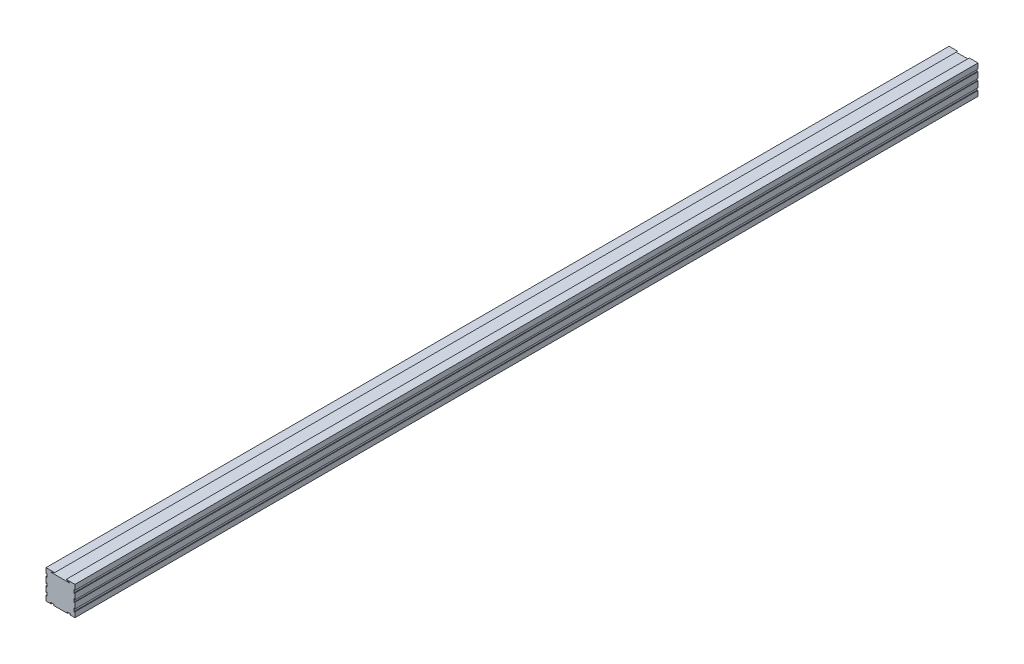
SolidWorks part; units mm, degrees
ref_plane "前视基准面" through (0, 0, 0) normal (0, 0, 1) x (1, 0, 0)
ref_plane "上视基准面" through (0, 0, 0) normal (0, 1, 0) x (1, 0, 0)
ref_plane "右视基准面" through (0, 0, 0) normal (1, 0, 0) x (0, 0, -1)
sketch "草图1" plane through (0, 0, 0) normal (0, 0, 1) x (1, 0, 0)
  line L1 (-37.5, 37.5) -> (37.5, 37.5)
  line L2 (-37.5, 37.5) -> (-37.5, -37.5)
  line L3 (-37.5, -37.5) -> (37.5, -37.5)
  line L4 (37.5, 37.5) -> (37.5, -37.5)
  line L5 (-37.5, 37.5) -> (37.5, -37.5) construction
  line L6 (-37.5, -37.5) -> (37.5, 37.5) construction
  point P0 (0, 0)
  dimension "D1" = 75
  dimension "D2" = 75
extrude "凸台-拉伸1" add sketch "草图1" along normal mid plane 2340 contours L1 L4 L3 L2
sketch "草图2" plane through (0, 0, 0) normal (0, 0, 1) x (1, 0, 0)
  line L0 (-37.5, -37.5) -> (37.5, -37.5) construction
  line L1 (-17.9, -36.8) -> (-16.55, -36.8)
  line L2 (-24.1, -36.8) -> (-24.1, -37.5)
  line L3 (-24.1, -37.5) -> (-17.9, -37.5)
  line L4 (-17.9, -36.8) -> (-17.9, -37.5)
  line L5 (-21, -38.432) -> (-21, -32.3332) construction
  line L6 (-25.45, -34.5) -> (-16.55, -34.5)
  line L7 (-25.45, -34.5) -> (-25.45, -36.8)
  line L8 (-25.45, -36.8) -> (-24.1, -36.8)
  line L9 (-16.55, -34.5) -> (-16.55, -36.8)
  line L10 (0, -20.0698) -> (0, -49.6644) construction
  line L11 (21, -38.432) -> (21, -32.3332) construction
  line L12 (16.55, -34.5) -> (16.55, -36.8)
  line L13 (25.45, -36.8) -> (24.1, -36.8)
  line L14 (25.45, -34.5) -> (25.45, -36.8)
  line L15 (25.45, -34.5) -> (16.55, -34.5)
  line L16 (17.9, -36.8) -> (17.9, -37.5)
  line L17 (24.1, -37.5) -> (17.9, -37.5)
  line L18 (24.1, -36.8) -> (24.1, -37.5)
  line L19 (17.9, -36.8) -> (16.55, -36.8)
  dimension "D1" = 6.2
  dimension "D2" = 8.9
  dimension "D3" = 0.7
  dimension "D4" = 2.3
  dimension "D5" = 3.1
  dimension "D6" = 4.45
  dimension "D7" = 21
extrude "切除-拉伸1" cut sketch "草图2" against normal mid plane 2340
sketch "草图3" plane through (0, 0, 1170) normal (0, 0, 1) x (1, 0, 0)
  line L0 (37.5, 37.5) -> (37.5, -37.5) construction
  line L1 (37.5, 2.6) -> (36.8, 2.6)
  line L2 (37.5, 2.6) -> (37.5, -2.6)
  line L3 (37.5, -2.6) -> (36.8, -2.6)
  line L4 (36.8, -2.6) -> (36.8, -4.45)
  line L5 (0, 0) -> (42.093, 0) construction
  line L6 (34.5, 4.45) -> (36.8, 4.45)
  line L7 (34.5, 4.45) -> (34.5, -4.45)
  line L8 (34.5, -4.45) -> (36.8, -4.45)
  line L9 (36.8, 4.45) -> (36.8, 2.6)
  line L10 (39.5858, -21) -> (29.5778, -21) construction
  line L11 (37.5, -17.9) -> (36.8, -17.9)
  line L12 (37.5, -17.9) -> (37.5, -24.1)
  line L13 (37.5, -24.1) -> (36.8, -24.1)
  line L14 (39.5858, 21) -> (29.5778, 21) construction
  line L15 (34.5, -16.55) -> (36.8, -16.55)
  line L16 (34.5, -16.55) -> (34.5, -25.45)
  line L17 (34.5, -25.45) -> (36.8, -25.45)
  line L18 (36.8, -16.55) -> (36.8, -17.9)
  line L19 (36.8, -24.1) -> (36.8, -25.45)
  line L20 (36.8, 24.1) -> (36.8, 25.45)
  line L21 (36.8, 16.55) -> (36.8, 17.9)
  line L22 (34.5, 25.45) -> (36.8, 25.45)
  line L23 (34.5, 16.55) -> (34.5, 25.45)
  line L24 (34.5, 16.55) -> (36.8, 16.55)
  line L25 (37.5, 24.1) -> (36.8, 24.1)
  line L26 (37.5, 17.9) -> (37.5, 24.1)
  line L27 (37.5, 17.9) -> (36.8, 17.9)
  line L28 (0, 28.4328) -> (0, -27.557) construction
  dimension "D1" = 5.2
  dimension "D2" = 2.6
  dimension "D3" = 8.9
  dimension "D4" = 4.45
  dimension "D5" = 0.7
  dimension "D6" = 2.3
  dimension "D7" = 6.2
  dimension "D8" = 8.9
  dimension "D9" = 3.1
  dimension "D10" = 4.45
  dimension "D11" = 0.7
  dimension "D12" = 2.3
  dimension "D13" = 21
extrude "切除-拉伸2" cut sketch "草图3" against normal blind 2340
mirror "镜向1" about plane through (0, 0, 0) normal (1, 0, 0) of "切除-拉伸2"
sketch "草图4" plane through (0, 0, 1170) normal (0, 0, 1) x (1, 0, 0)
  line L0 (-15, 37.5) -> (-25, 33.5)
  line L1 (-37.5, 37.5) -> (37.5, 37.5) construction
  line L2 (-25, 33.5) -> (25, 33.5)
  line L3 (25, 33.5) -> (15, 37.5)
  dimension "D1" = 50
  dimension "D2" = 25
  dimension "D3" = 30
  dimension "D4" = 15
  dimension "D5" = 4
extrude "切除-拉伸3" cut sketch "草图4" against normal through all and the other way through all
